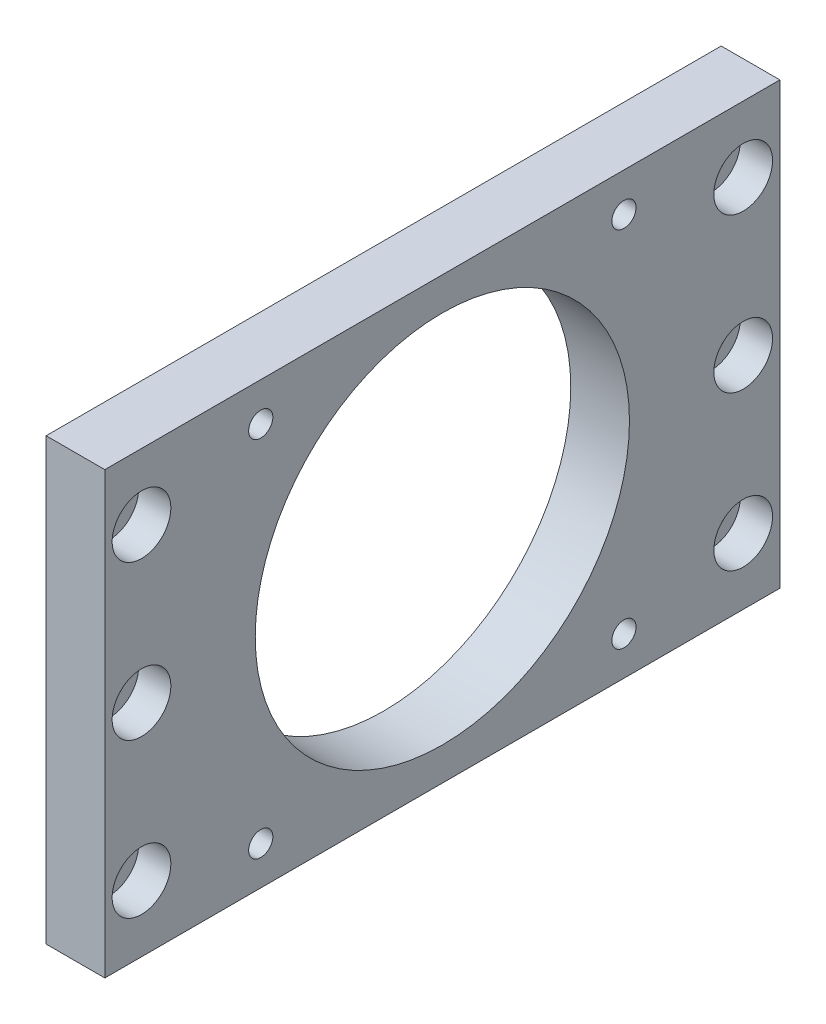
from build123d import *

# Parameters (mm, degrees)
SKETCH1_W                                           = 92
SKETCH1_H                                           = 60
BOSS_EXTRUDE1_DEPTH                                 = 4
M4_TAPPED_HOLE1_D                                   = 3.3
M4_TAPPED_HOLE1_DEPTH                               = 10.1
M4_TAPPED_HOLE1_TIP                                 = 0.991420021
SKETCH4_R                                           = 25.5
CUT_EXTRUDE1_DEPTH                                  = 56.497747702
CBORE_FOR_M4_HEX_SOCKET_HEAD_CAP_SCREW1_D           = 4.5
CBORE_FOR_M4_HEX_SOCKET_HEAD_CAP_SCREW1_CBORE_D     = 8
CBORE_FOR_M4_HEX_SOCKET_HEAD_CAP_SCREW1_CBORE_DEPTH = 4.4
M4_TAPPED_HOLE2_D                                   = 3.3
M4_TAPPED_HOLE2_DEPTH                               = 10.1
M4_TAPPED_HOLE2_TIP                                 = 0.991420021


with BuildPart() as part:
    # Sketch1 → Boss-Extrude1 (new, symmetric)
    with BuildSketch(Plane(origin=(0, 0, 0), x_dir=(0, 0, -1), z_dir=(1, 0, 0))):
        Rectangle(SKETCH1_W, SKETCH1_H)
    extrude(amount=BOSS_EXTRUDE1_DEPTH, both=True)

    # M4 Tapped Hole1
    with Locations(Plane(origin=(4, 0, 0), x_dir=(0, 0, -1), z_dir=(1, 0, 0))):
        with Locations((-24.75, 24.75), (24.75, 24.75), (-24.75, -24.75), (24.75, -24.75)):
            Hole(M4_TAPPED_HOLE1_D / 2, depth=M4_TAPPED_HOLE1_DEPTH)
            with Locations((0, 0, -(M4_TAPPED_HOLE1_DEPTH + M4_TAPPED_HOLE1_TIP / 2))):  # 118° drill point
                Cone(0, M4_TAPPED_HOLE1_D / 2, M4_TAPPED_HOLE1_TIP, mode=Mode.SUBTRACT)

    # Sketch4 → Cut-Extrude1 (cut, through all)
    with BuildSketch(Plane(origin=(4, 0, 0), x_dir=(0, 0, -1), z_dir=(1, 0, 0))):
        Circle(SKETCH4_R)
    extrude(amount=-CUT_EXTRUDE1_DEPTH, mode=Mode.SUBTRACT)

    # CBORE for M4 Hex Socket Head Cap Screw1 (through all)
    with Locations(Plane(origin=(4, 0, 0), x_dir=(0, 0, -1), z_dir=(1, 0, 0))):
        with Locations((-41, 21), (-41, 0), (-41, -21), (41, 21), (41, 0), (41, -21)):
            CounterBoreHole(CBORE_FOR_M4_HEX_SOCKET_HEAD_CAP_SCREW1_D / 2, CBORE_FOR_M4_HEX_SOCKET_HEAD_CAP_SCREW1_CBORE_D / 2, CBORE_FOR_M4_HEX_SOCKET_HEAD_CAP_SCREW1_CBORE_DEPTH)

    # M4 Tapped Hole2
    with Locations(Plane(origin=(0, -30, 0), x_dir=(-1, 0, 0), z_dir=(0, -1, 0))):
        with Locations((0, -34), (0, 34)):
            Hole(M4_TAPPED_HOLE2_D / 2, depth=M4_TAPPED_HOLE2_DEPTH)
            with Locations((0, 0, -(M4_TAPPED_HOLE2_DEPTH + M4_TAPPED_HOLE2_TIP / 2))):  # 118° drill point
                Cone(0, M4_TAPPED_HOLE2_D / 2, M4_TAPPED_HOLE2_TIP, mode=Mode.SUBTRACT)


solid = part.part
